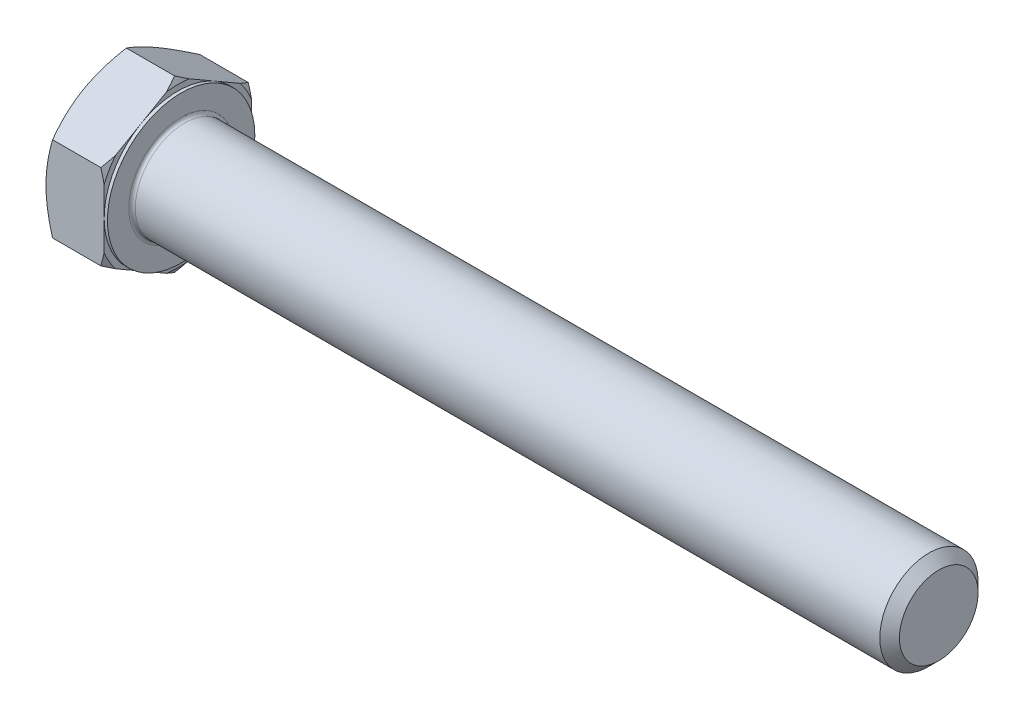
from build123d import *

# Parameters (mm, degrees)
BASE_EXTRUDE_DEPTH = 15
SKETCH4_W          = 0.8
SKETCH4_H          = 12.784609691
CHAMFER_2_SIZE     = 2.4
FILLET_2_R         = 0.8


with BuildPart() as part:
    # Sketch1 → Base-Extrude (new body)
    with BuildSketch(Plane(origin=(0, 0, 0), x_dir=(0, 0, -1), z_dir=(1, 0, 0))):
        Polygon((18, 10.392304845), (18, -10.392304845), (0, -20.784609691), (-18, -10.392304845), (-18, 10.392304845), (0, 20.784609691), align=None)
    extrude(amount=BASE_EXTRUDE_DEPTH)

    # Sketch2 → Boss-Revolve1 (revolve)
    with BuildSketch(Plane.XY, mode=Mode.PRIVATE) as boss_revolve1_sk:
        Polygon((0, 0), (200, 0), (200, 9.402), (200, 12), (27.8072, 12), (0, 12), align=None)
    revolve(boss_revolve1_sk.sketch.rotate(Axis((0, 0, 0), (1, 0, 0)), 90), axis=Axis((0, 0, 0), (1, 0, 0)))

    # Sketch3 → Cut-Revolve1 (revolve, cut)
    with BuildSketch(Plane.XY):
        Polygon((0, 18), (4.494446501, 25.784609691), (4.494446501, 30.784609691), (-10, 30.784609691), (-10, 18), align=None)
    revolve(axis=Axis((0, 0, 0), (1, 0, 0)), mode=Mode.SUBTRACT)

    # Sketch5 → Cut-Revolve2 (revolve, cut)
    with BuildSketch(Plane.XY):
        Polygon((15, 18), (10.505553499, 25.784609691), (10.505553499, 30.784609691), (20.505553499, 30.784609691), (20.505553499, 18), align=None)
    revolve(axis=Axis((0, 0, 0), (1, 0, 0)), mode=Mode.SUBTRACT)

    # Sketch4 → Cut-Revolve3 (revolve, cut)
    with BuildSketch(Plane.XY, mode=Mode.PRIVATE) as cut_revolve3_sk:
        with Locations((14.6, 24.392304845)):
            Rectangle(SKETCH4_W, SKETCH4_H)
    revolve(cut_revolve3_sk.sketch.rotate(Axis((0, 0, 0), (1, 0, 0)), 270), axis=Axis((0, 0, 0), (1, 0, 0)), mode=Mode.SUBTRACT)

    # Chamfer 2
    chamfer_2_edges = [part.edges().sort_by_distance(p)[0] for p in [
        (200, 0, -12),
    ]]
    chamfer(chamfer_2_edges, length=CHAMFER_2_SIZE)

    # Fillet 2
    fillet_2_edges = [part.edges().sort_by_distance(p)[0] for p in [
        (15, 0, -12),
    ]]
    fillet(fillet_2_edges, radius=FILLET_2_R)


solid = part.part
